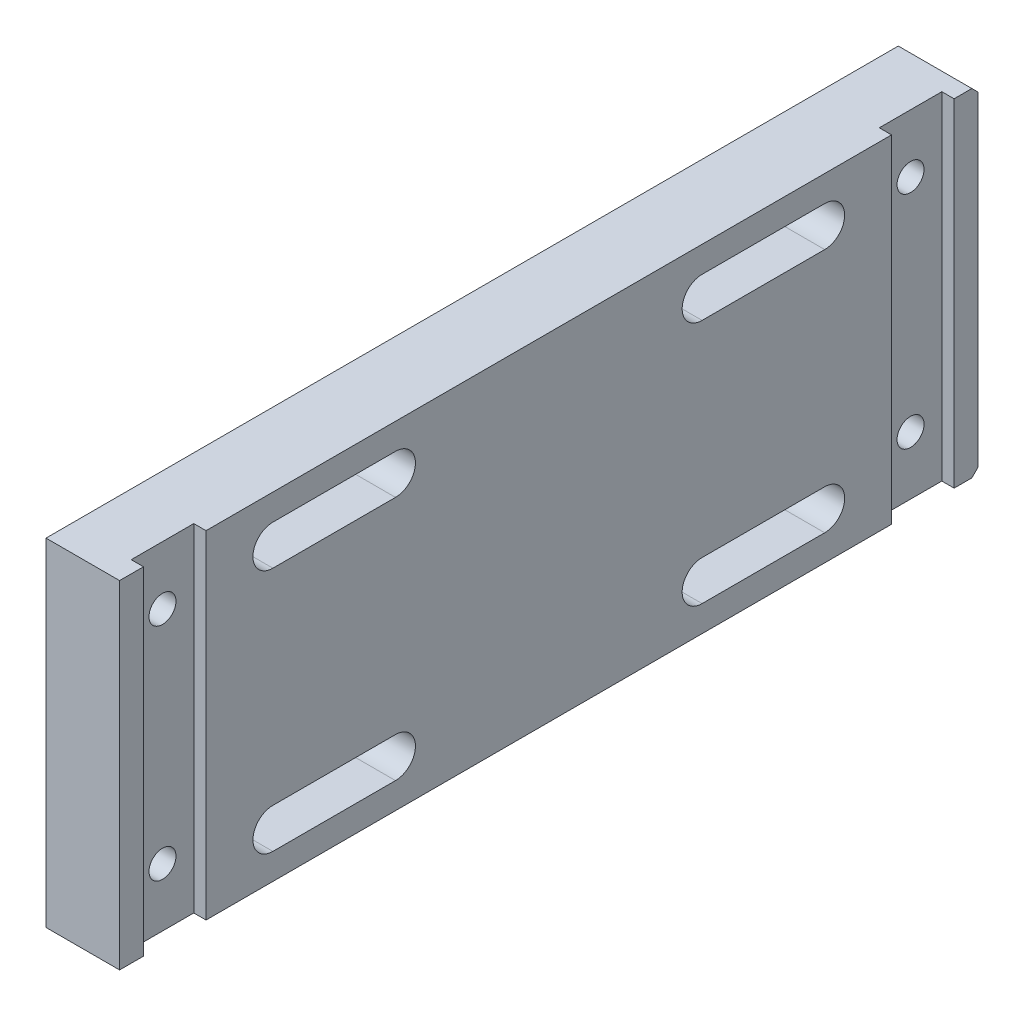
SolidWorks part; units mm, degrees
material "6061铝"
ref_plane "前视基准面" through (0, 0, 0) normal (0, 0, 1) x (1, 0, 0)
ref_plane "上视基准面" through (0, 0, 0) normal (0, 1, 0) x (1, 0, 0)
ref_plane "右视基准面" through (0, 0, 0) normal (1, 0, 0) x (0, 0, -1)
sketch "草图1" plane through (0, 0, 0) normal (1, 0, 0) x (0, 0, -1)
  line L1 (-70, 27.5) -> (70, 27.5)
  line L2 (-70, 27.5) -> (-70, -27.5)
  line L3 (-70, -27.5) -> (70, -27.5)
  line L4 (70, 27.5) -> (70, -27.5)
  line L5 (-70, 27.5) -> (70, -27.5) construction
  line L6 (-70, -27.5) -> (70, 27.5) construction
  point P0 (0, 0)
  dimension "D1" = 55
  dimension "D2" = 140
extrude "凸台-拉伸1" add sketch "草图1" along normal blind 12
sketch "草图2" plane through (12, 0, 0) normal (1, 0, 0) x (0, 0, -1)
  line L1 (-66.1, 33.3411) -> (-55.9, 33.3411)
  line L2 (-66.1, 33.3411) -> (-66.1, -34.4007)
  line L3 (-66.1, -34.4007) -> (-55.9, -34.4007)
  line L4 (-55.9, 33.3411) -> (-55.9, -34.4007)
  line L5 (-66.1, 33.3411) -> (-55.9, -34.4007) construction
  line L6 (-66.1, -34.4007) -> (-55.9, 33.3411) construction
  point P0 (-61, -0.5298)
  dimension "D1" = 10.2
  dimension "D3" = 61
extrude "切除-拉伸1" cut sketch "草图2" against normal blind 2
chamfer "倒角1" distance 1 angle 45 2 edges at (6, -27.5, -70) (6, 27.5, -70)
mirror "镜向2" about plane through (0, 0, 0) normal (0, 0, 1) of "切除-拉伸1"
sketch "草图3" plane through (12, 0, 0) normal (1, 0, 0) x (0, 0, -1)
  line L0 (-45, 20) -> (-25, 20) construction
  line L1 (-45, 23.25) -> (-25, 23.25)
  line L2 (-45, 16.75) -> (-25, 16.75)
  line L3 (-35, 20) -> (-35, -33.5115) construction
  line L4 (0, 0) -> (0, 38.3818) construction
  line L5 (0, 0) -> (-64.5605, 0) construction
  line L6 (-45, -20) -> (-25, -20) construction
  line L7 (-45, -23.25) -> (-25, -23.25)
  line L8 (-45, -16.75) -> (-25, -16.75)
  line L9 (45, 20) -> (25, 20) construction
  line L10 (45, 23.25) -> (25, 23.25)
  line L11 (45, 16.75) -> (25, 16.75)
  line L12 (45, -20) -> (25, -20) construction
  line L13 (45, -23.25) -> (25, -23.25)
  line L14 (45, -16.75) -> (25, -16.75)
  arc A0 (-45, 23.25) -> (-45, 16.75) centre (-45, 20) ccw
  arc A1 (-25, 16.75) -> (-25, 23.25) centre (-25, 20) ccw
  arc A2 (-45, -23.25) -> (-45, -16.75) centre (-45, -20) cw
  arc A3 (-25, -16.75) -> (-25, -23.25) centre (-25, -20) cw
  arc A4 (45, 23.25) -> (45, 16.75) centre (45, 20) cw
  arc A5 (25, 16.75) -> (25, 23.25) centre (25, 20) cw
  arc A6 (45, -23.25) -> (45, -16.75) centre (45, -20) ccw
  arc A7 (25, -16.75) -> (25, -23.25) centre (25, -20) ccw
  point P2 (-35, 20)
  point P15 (-35, -20)
  point P22 (35, 20)
  point P29 (35, -20)
  dimension "D1" = 3.25
  dimension "D2" = 20
  dimension "D3" = 40
  dimension "D4" = 70
extrude "切除-拉伸2" cut sketch "草图3" against normal blind 36
hole_wizard "打孔尺寸(%根据)内六角圆柱头螺钉的类型0" positions "草图4" profile "草图6" counterbore size "M4" standard "GB" end condition through all
sketch "草图4" plane through (0, 0, 0) normal (-1, 0, 0) x (0, 0, 1)
  point P6 (-61, 18)
  point P9 (-61, -18)
  point P13 (61, 18)
  point P16 (61, -18)
sketch "草图6" plane through (0, 18, -61) normal (0, 1, 0) x (0, 0, 1)
  line L0 (0, 0) -> (0, 12)
  line L1 (0, 12) -> (2.2, 12)
  line L3 (2.2, 12) -> (2.2, 5)
  line L4 (2.2, 5) -> (4, 5)
  line L5 (4, 5) -> (4, 0)
  line L7 (4, 0) -> (0, 0)
  line L11 (0, -6.35) -> (0, 107.95) construction
  dimension "通孔孔直径" = 4.4
  dimension "通孔孔深度" = 12
  dimension "柱形沉头孔直径" = 8
  dimension "柱形沉头孔深度" = 5
